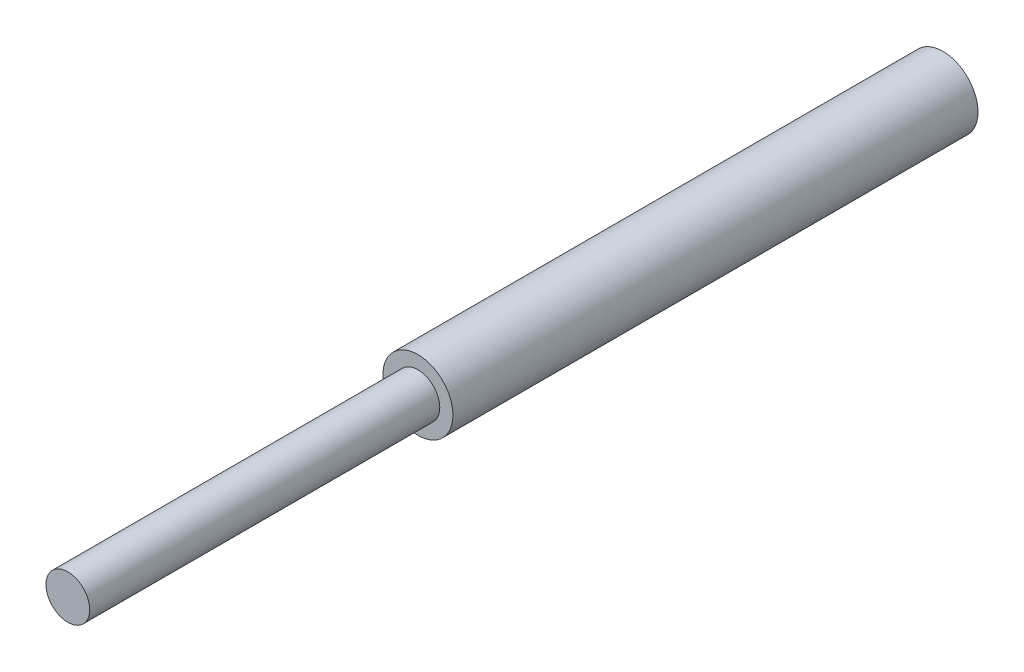
from build123d import *

# Parameters (mm, degrees)
SKETCH_1_R          = 4
EXTRUDE_1_DEPTH     = 100
CUT_EXTRUDE_START   = -40
SKETCH_2_R          = 4
SKETCH_2_R_2        = 2.5
CUT_EXTRUDE_1_DEPTH = 40


with BuildPart() as part:
    # 草图1 → 凸台-拉伸1 (new body)
    with BuildSketch(Plane.XY):
        Circle(SKETCH_1_R)
    extrude(amount=EXTRUDE_1_DEPTH)

    # 草图2 → 切除-拉伸1 (cut)
    with BuildSketch(Plane.XY.offset(100).offset(CUT_EXTRUDE_START)):
        Circle(SKETCH_2_R)
        Circle(SKETCH_2_R_2, mode=Mode.SUBTRACT)
    extrude(amount=CUT_EXTRUDE_1_DEPTH, mode=Mode.SUBTRACT)


solid = part.part
